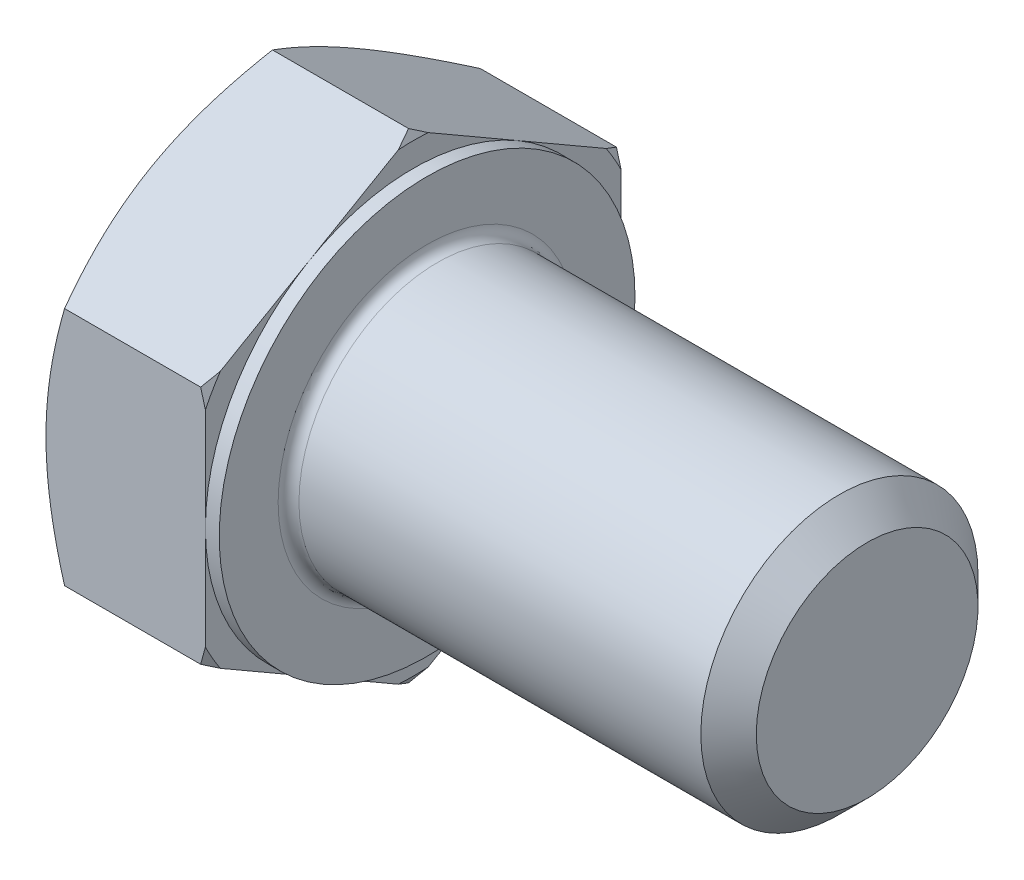
from build123d import *

# Parameters (mm, degrees)
BASE_EXTRUDE_DEPTH = 10
SKETCH4_W          = 0.8
SKETCH4_H          = 11.856406461
CHAMFER_2_SIZE     = 1.6
FILLET_2_R         = 0.6


with BuildPart() as part:
    # Sketch1 → Base-Extrude (new body)
    with BuildSketch(Plane(origin=(0, 0, 0), x_dir=(0, 0, -1), z_dir=(1, 0, 0))):
        Polygon((12, 6.92820323), (12, -6.92820323), (0, -13.856406461), (-12, -6.92820323), (-12, 6.92820323), (0, 13.856406461), align=None)
    extrude(amount=BASE_EXTRUDE_DEPTH)

    # Sketch2 → Boss-Revolve1 (revolve)
    with BuildSketch(Plane.XY, mode=Mode.PRIVATE) as boss_revolve1_sk:
        Polygon((0, 0), (35.4, 0), (35.4, 6.268), (35.4, 8), (27.8072, 8), (0, 8), align=None)
    revolve(boss_revolve1_sk.sketch.rotate(Axis((0, 0, 0), (1, 0, 0)), 90), axis=Axis((0, 0, 0), (1, 0, 0)))

    # Sketch3 → Cut-Revolve1 (revolve, cut)
    with BuildSketch(Plane.XY):
        Polygon((0, 12), (3.958548116, 18.856406461), (3.958548116, 23.856406461), (-10, 23.856406461), (-10, 12), align=None)
    revolve(axis=Axis((0, 0, 0), (1, 0, 0)), mode=Mode.SUBTRACT)

    # Sketch5 → Cut-Revolve2 (revolve, cut)
    with BuildSketch(Plane.XY):
        Polygon((10, 12), (6.041451884, 18.856406461), (6.041451884, 23.856406461), (16.041451884, 23.856406461), (16.041451884, 12), align=None)
    revolve(axis=Axis((0, 0, 0), (1, 0, 0)), mode=Mode.SUBTRACT)

    # Sketch4 → Cut-Revolve3 (revolve, cut)
    with BuildSketch(Plane.XY, mode=Mode.PRIVATE) as cut_revolve3_sk:
        with Locations((9.6, 17.928203231)):
            Rectangle(SKETCH4_W, SKETCH4_H)
    revolve(cut_revolve3_sk.sketch.rotate(Axis((0, 0, 0), (1, 0, 0)), 270), axis=Axis((0, 0, 0), (1, 0, 0)), mode=Mode.SUBTRACT)

    # Chamfer 2
    chamfer_2_edges = [part.edges().sort_by_distance(p)[0] for p in [
        (35.4, 0, -8),
    ]]
    chamfer(chamfer_2_edges, length=CHAMFER_2_SIZE)

    # Fillet 2
    fillet_2_edges = [part.edges().sort_by_distance(p)[0] for p in [
        (10, 0, -8),
    ]]
    fillet(fillet_2_edges, radius=FILLET_2_R)


solid = part.part
